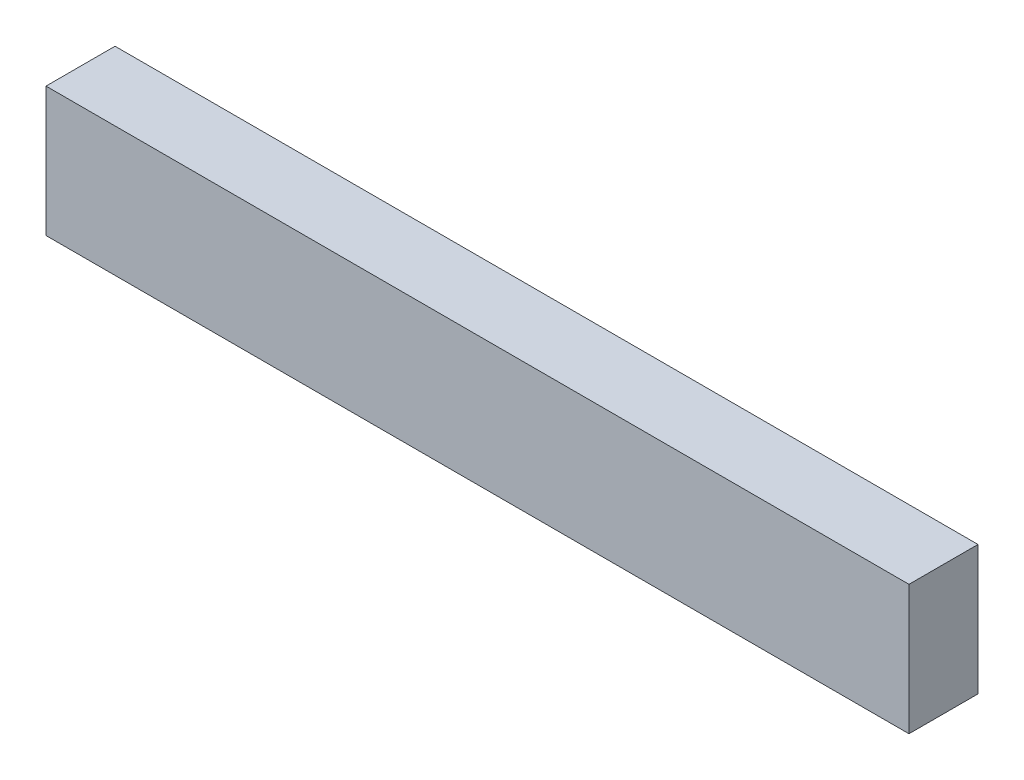
from build123d import *

# Parameters (mm, degrees)
SKETCH_1_W      = 100
SKETCH_1_H      = 15
EXTRUDE_1_DEPTH = 8


with BuildPart() as part:
    # 草图1 → 凸台-拉伸1 (new body)
    with BuildSketch(Plane.XY):
        Rectangle(SKETCH_1_W, SKETCH_1_H)
    extrude(amount=EXTRUDE_1_DEPTH)


solid = part.part
